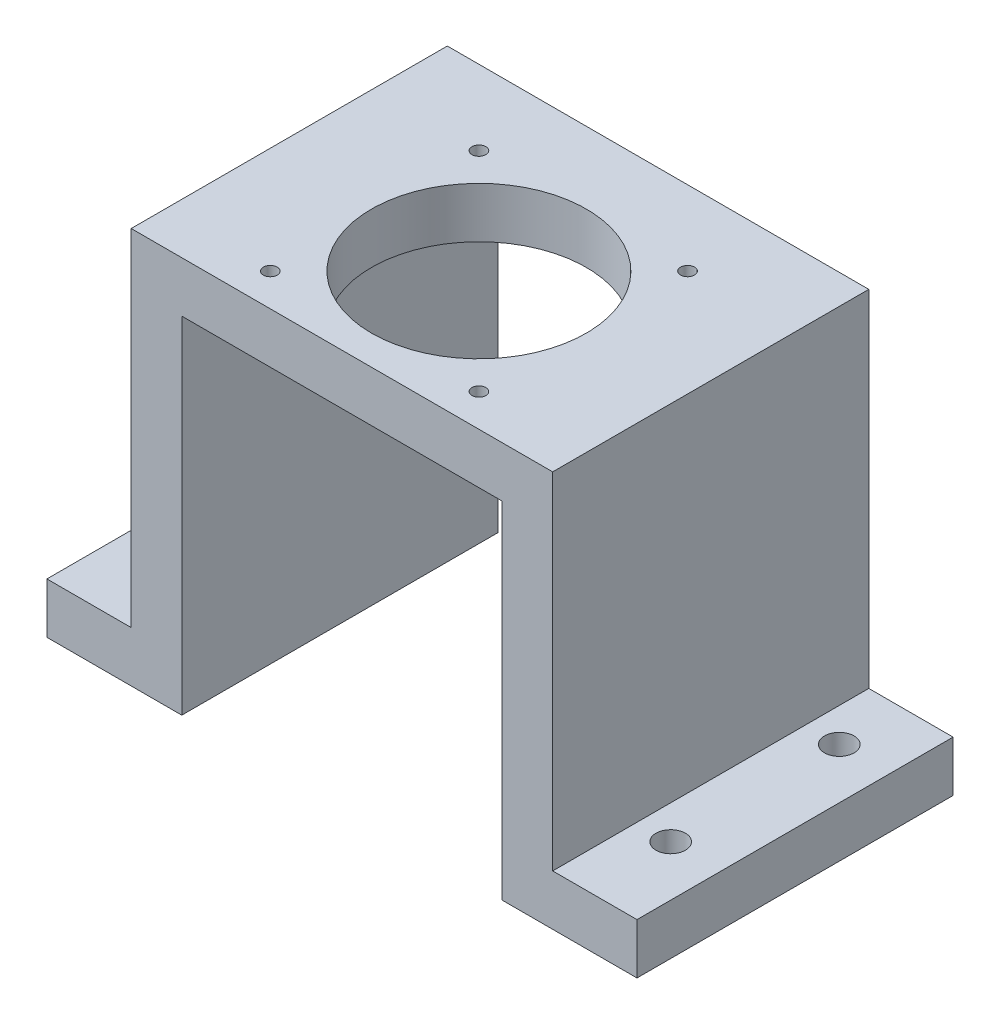
SolidWorks part; units mm, degrees
ref_plane "Front Plane" through (0, 0, 0) normal (0, 0, 1) x (1, 0, 0)
ref_plane "Top Plane" through (0, 0, 0) normal (0, 1, 0) x (1, 0, 0)
ref_plane "Right Plane" through (0, 0, 0) normal (1, 0, 0) x (0, 0, -1)
sketch "Sketch1" plane through (0, 0, 0) normal (0, 0, 1) x (1, 0, 0)
  line L0 (-70, 0) -> (-50, 0)
  line L1 (-50, 0) -> (-50, 82)
  line L2 (-50, 82) -> (50, 82)
  line L3 (50, 82) -> (50, 0)
  line L4 (50, 0) -> (70, 0)
  line L5 (0, 0) -> (22.0296, 0) construction
  line L6 (0, 0) -> (0, 80.4772) construction
  dimension "D1" = 100
  dimension "D2" = 20
  dimension "D3" = 82
extrude "Extrude-Thin1" add sketch "Sketch1" along normal blind 75 thin
sketch "Sketch2" plane through (0, 82, 0) normal (0, 1, 0) x (1, 0, 0)
  line L0 (0, 0) -> (0, -105.0434) construction
  line L1 (-50, 0) -> (50, 0) construction
  circle A0 centre (0, -42.5) radius 25.5
  dimension "D1" = 51
  dimension "D2" = 42.5
extrude "Cut-Extrude1" cut sketch "Sketch2" against normal through all
sketch "Sketch4" plane through (0, 0, 0) normal (0, 1, 0) x (1, 0, 0)
  line L0 (0, 0) -> (0, 43.6534) construction
  line L3 (-70, 0) -> (-50, 0) construction
  circle A0 centre (-58, -15) radius 3.5
  circle A1 centre (58, -15) radius 3.5
  circle A2 centre (58, -55) radius 3.5
  circle A3 centre (-58, -55) radius 3.5
  dimension "D1" = 40
  dimension "D2" = 58
  dimension "D3" = 7
  dimension "D4" = 15
extrude "Cut-Extrude3" cut sketch "Sketch4" against normal through all
hole_wizard "M4 Tapped Hole1" positions "Sketch6" profile "Sketch5" tap size "M4" standard "Gb" end condition through all
sketch "Sketch6" plane through (0, 82, 0) normal (0, 1, 0) x (1, 0, 0)
  line L0 (0, -42.5) -> (-24.7487, -17.7513) construction
  line L2 (0, -42.5) -> (0, 21.9121) construction
  circle A0 centre (0, -42.5) radius 35 construction
  circle A1 centre (0, -42.5) radius 35 construction
  circle A2 centre (0, -42.5) radius 35 construction
  circle A3 centre (0, -42.5) radius 35 construction
  point P0 (-24.7487, -17.7513)
  point P42 (24.7487, -17.7513)
  point P44 (24.7487, -67.2487)
  point P46 (-24.7487, -67.2487)
  dimension "D1" = 70
  dimension "D2" = 45
  dimension "D3" = 4
cosmetic thread "Cosmetic Thread7" parameters "D2"=4
cosmetic thread "Cosmetic Thread8" parameters "D2"=4
cosmetic thread "Cosmetic Thread9" parameters "D2"=4
cosmetic thread "Cosmetic Thread10" parameters "D2"=4
sketch "Sketch5" plane through (-24.7487, 82, 17.7513) normal (1, 0, 0) x (0, 0, 1)
  line L0 (0, 0) -> (0, 94)
  line L1 (0, 94) -> (1.65, 94)
  line L2 (1.65, 94) -> (1.65, 0)
  line L5 (1.65, 0) -> (0, 0)
  line L11 (0, -6.35) -> (0, 107.95) construction
  dimension "通孔螺纹孔钻头直径" = 3.3
  dimension "通孔螺纹孔钻头深度" = 94
